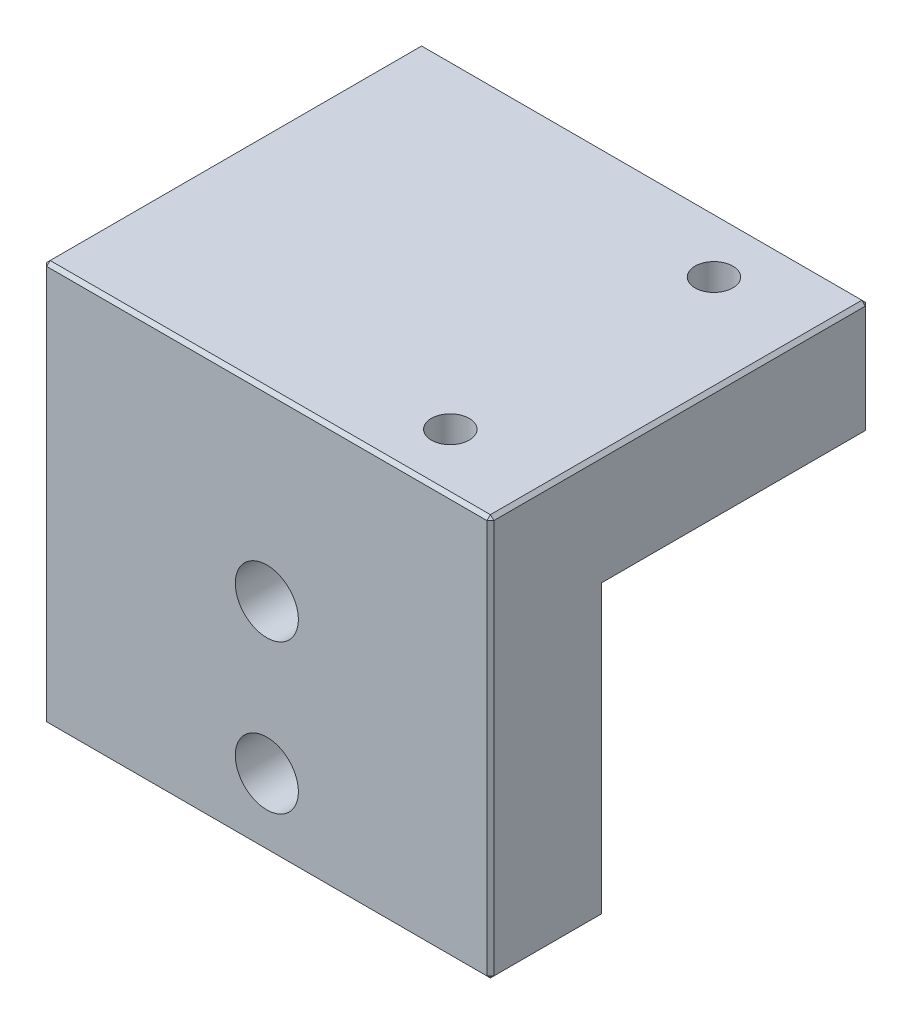
from build123d import *

# Parameters (mm, degrees)
SKETCH_1_W                   = 39
SKETCH_1_H                   = 33
EXTRUDE_1_DEPTH              = 10
SKETCH_2_W                   = 39
SKETCH_2_H                   = 10
EXTRUDE_2_DEPTH              = 25
HOLE_WIZARD_M4_1_D           = 3.3
HOLE_WIZARD_M4_1_DEPTH       = 13.5
HOLE_WIZARD_M4_1_TIP         = 0.991420021
HOLE_WIZARD_M5_1_D           = 5.5
HOLE_WIZARD_M5_1_CBORE_D     = 10
HOLE_WIZARD_M5_1_CBORE_DEPTH = 5.4
CHAMFER_1_SIZE               = 0.3


with BuildPart() as part:
    # 草图1 → 凸台-拉伸1 (new body)
    with BuildSketch(Plane(origin=(0, 0, 0), x_dir=(1, 0, 0), z_dir=(0, 1, 0))):
        Rectangle(SKETCH_1_W, SKETCH_1_H)
    extrude(amount=EXTRUDE_1_DEPTH)

    # 草图2 → 凸台-拉伸2 (add)
    with BuildSketch(Plane.XZ):
        with Locations((0, 11.5)):
            Rectangle(SKETCH_2_W, SKETCH_2_H)
    extrude(amount=EXTRUDE_2_DEPTH)

    # M4 螺纹孔1
    with Locations(Plane(origin=(0, 10, 0), x_dir=(1, 0, 0), z_dir=(0, 1, 0))):
        with Locations((11, 11.5), (11, -11.5)):
            Hole(HOLE_WIZARD_M4_1_D / 2, depth=HOLE_WIZARD_M4_1_DEPTH)
            with Locations((0, 0, -(HOLE_WIZARD_M4_1_DEPTH + HOLE_WIZARD_M4_1_TIP / 2))):  # 118° drill point
                Cone(0, HOLE_WIZARD_M4_1_D / 2, HOLE_WIZARD_M4_1_TIP, mode=Mode.SUBTRACT)

    # M5 六角凹头螺钉的柱形沉头孔1 (through all)
    with Locations(Plane(origin=(0, 0, 6.5), x_dir=(-1, 0, 0), z_dir=(0, 0, -1))):
        with Locations((0, -6), (0, -19)):
            CounterBoreHole(HOLE_WIZARD_M5_1_D / 2, HOLE_WIZARD_M5_1_CBORE_D / 2, HOLE_WIZARD_M5_1_CBORE_DEPTH)

    # 倒角1
    chamfer_1_edges = [part.edges().sort_by_distance(p)[0] for p in [
        (0, -25, 16.5),
        (0, -25, 6.5),
        (0, 10, -16.5),
        (0, 0, -16.5),
        (-19.5, 5, -16.5),
        (-19.5, 10, 0),
        (-19.5, 0, -5),
        (-19.5, -12.5, 6.5),
        (-19.5, -25, 11.5),
        (-19.5, -7.5, 16.5),
        (19.5, 10, 0),
        (19.5, 5, -16.5),
        (19.5, 0, -5),
        (19.5, -12.5, 6.5),
        (19.5, -25, 11.5),
        (19.5, -7.5, 16.5),
        (0, 10, 16.5),
    ]]
    chamfer(chamfer_1_edges, length=CHAMFER_1_SIZE)


solid = part.part
